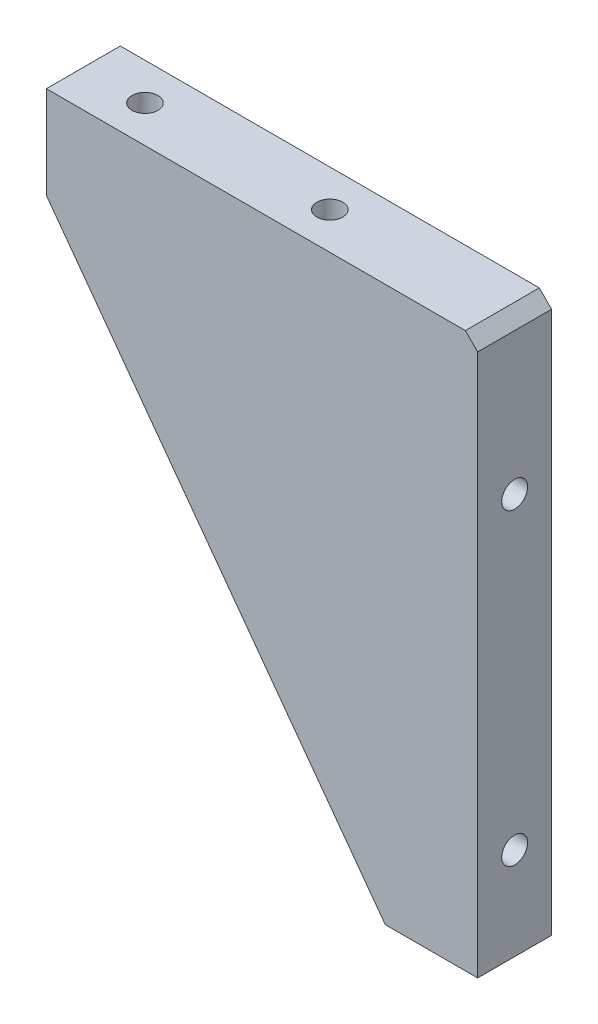
from build123d import *

# Parameters (mm, degrees)
EXTRUDE_1_DEPTH        = 12
HOLE_WIZARD_M5_1_D     = 4.2
HOLE_WIZARD_M5_1_DEPTH = 12.4
HOLE_WIZARD_M5_1_TIP   = 1.2618073
HOLE_WIZARD_M5_2_D     = 4.2
HOLE_WIZARD_M5_2_DEPTH = 12.4
HOLE_WIZARD_M5_2_TIP   = 1.2618073
CHAMFER_1_SIZE         = 2


with BuildPart() as part:
    # 草图1 → 凸台-拉伸1 (new body)
    with BuildSketch(Plane.XY):
        Polygon((0, 0), (0, -90), (-15, -90), (-70, -15), (-70, 0), align=None)
    extrude(amount=EXTRUDE_1_DEPTH)

    # M5 螺纹孔1
    with Locations(Plane(origin=(0, 0, 0), x_dir=(1, 0, 0), z_dir=(0, 1, 0))):
        with Locations((-60, -6), (-30, -6)):
            Hole(HOLE_WIZARD_M5_1_D / 2, depth=HOLE_WIZARD_M5_1_DEPTH)
            with Locations((0, 0, -(HOLE_WIZARD_M5_1_DEPTH + HOLE_WIZARD_M5_1_TIP / 2))):  # 118° drill point
                Cone(0, HOLE_WIZARD_M5_1_D / 2, HOLE_WIZARD_M5_1_TIP, mode=Mode.SUBTRACT)

    # M5 螺纹孔2
    with Locations(Plane(origin=(0, 0, 0), x_dir=(0, 0, -1), z_dir=(1, 0, 0))):
        with Locations((-6, -75), (-6, -25)):
            Hole(HOLE_WIZARD_M5_2_D / 2, depth=HOLE_WIZARD_M5_2_DEPTH)
            with Locations((0, 0, -(HOLE_WIZARD_M5_2_DEPTH + HOLE_WIZARD_M5_2_TIP / 2))):  # 118° drill point
                Cone(0, HOLE_WIZARD_M5_2_D / 2, HOLE_WIZARD_M5_2_TIP, mode=Mode.SUBTRACT)

    # 倒角1
    chamfer_1_edges = [part.edges().sort_by_distance(p)[0] for p in [
        (0, 0, 6),
    ]]
    chamfer(chamfer_1_edges, length=CHAMFER_1_SIZE)


solid = part.part
